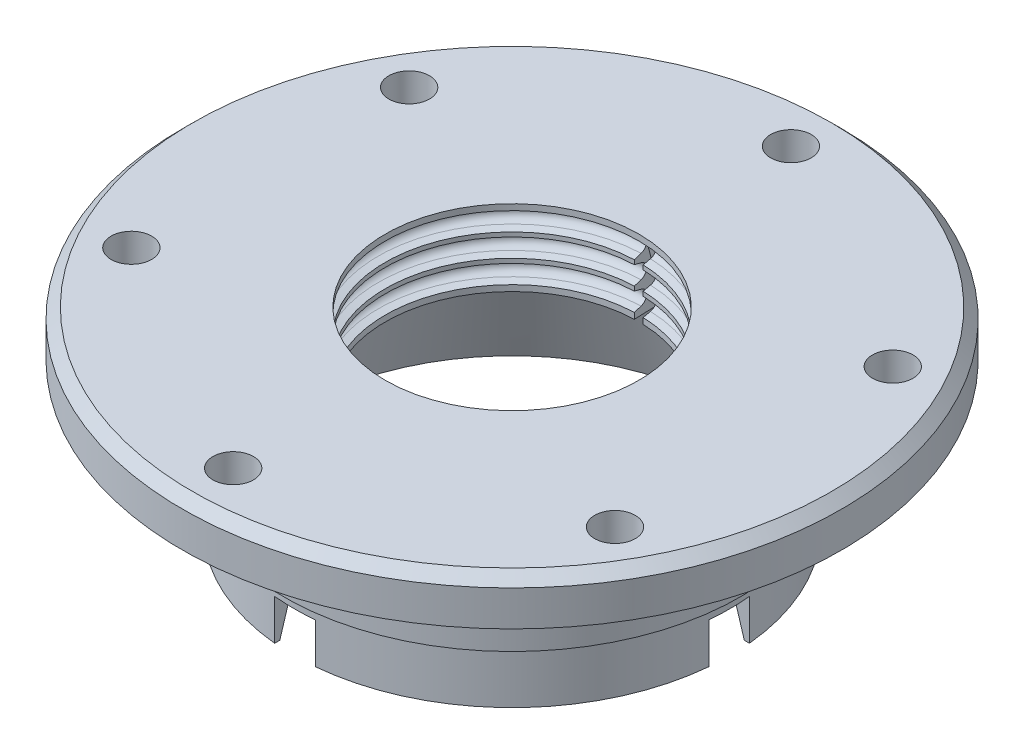
SolidWorks part; units mm, degrees
ref_plane "Front" through (0, 0, 0) normal (0, 0, 1) x (1, 0, 0)
ref_plane "Top" through (0, 0, 0) normal (0, 1, 0) x (1, 0, 0)
ref_plane "Right" through (0, 0, 0) normal (1, 0, 0) x (0, 0, -1)
sketch "Sketch1" plane through (0, 0, 0) normal (0, 0, 1) x (1, 0, 0)
  line L0 (-43, 0) -> (-43, 11)
  line L1 (-43, 11) -> (-45, 11)
  line L2 (-45, 11) -> (-45, 27)
  line L3 (-45, 27) -> (-43, 27)
  line L4 (-43, 27) -> (-43, 29)
  line L5 (-43, 29) -> (-65, 29)
  line L6 (-65, 29) -> (-65, 36)
  line L7 (-63, 38) -> (-25, 38)
  line L8 (-25, 33.1791) -> (-25, 32.3209) construction
  line L9 (-25, 23) -> (-35, 23)
  line L10 (-35, 23) -> (-42, 0)
  line L11 (-42, 0) -> (-43, 0)
  line L12 (-65, 36) -> (-63, 38)
  line L13 (-26, 43.5692) -> (-26, 24.4632) construction
  line L14 (-33.7723, 35) -> (-26, 35) construction
  line L15 (-33.7723, 30.5) -> (-26, 30.5) construction
  line L16 (-33.7723, 26) -> (-26, 26) construction
  line L17 (-26.3882, 36.4489) -> (-25, 36.8209)
  line L18 (-26.3882, 33.5511) -> (-25, 33.1791)
  line L19 (-26.3882, 31.9489) -> (-25, 32.3209)
  line L20 (-26.3882, 24.5511) -> (-25, 24.1791)
  line L21 (-26.5776, 27.3844) -> (-25, 27.8071)
  line L22 (-25, 28.6791) -> (-25, 27.8071) construction
  line L23 (-25, 24.1791) -> (-25, 15.722) construction
  line L24 (-25, 24.1791) -> (-25, 23)
  line L25 (-26.3882, 29.0511) -> (-25, 28.6791)
  line L26 (-25, 40.9901) -> (-25, 36.8209) construction
  line L27 (-25, 33.1791) -> (-25, 32.3209)
  line L28 (-25, 28.6791) -> (-25, 27.8071)
  line L29 (-25, 38) -> (-25, 36.8209)
  line L30 (0, 0) -> (0, 81.7826) construction
  arc A0 (-26.3882, 36.4489) -> (-26.3882, 33.5511) centre (-26, 35) ccw
  arc A1 (-26.3882, 31.9489) -> (-26.3882, 29.0511) centre (-26, 30.5) ccw
  arc A2 (-26.5776, 27.3844) -> (-26.3882, 24.5511) centre (-26, 26) ccw
  point P8 (-65, 38)
  dimension "D19" = 3
  dimension "D20" = 3
  dimension "D21" = 3
  dimension "D2" = 2
  dimension "D3" = 2
  dimension "D4" = 42
  dimension "D5" = 1
  dimension "D6" = 11
  dimension "D7" = 2
  dimension "D8" = 16
  dimension "D9" = 22
  dimension "D10" = 9
  dimension "D11" = 23
  dimension "D12" = 25
  dimension "D16" = 4.5
  dimension "D17" = 7.5
  dimension "D18" = 4.5
  dimension "D22" = 30
  dimension "D23" = 15
  dimension "D24" = 30
  dimension "D25" = 15
  dimension "D26" = 15
  dimension "D27" = 15
  dimension "D28" = 1
revolve "Revolve1" add sketch "Sketch1" angle 360 about L30
fillet "Fillet1" radius 5 1 edges at (0, 23, -35)
sketch "Sketch2" plane through (0, 0, 0) normal (0, 0, 1) x (1, 0, 0)
  line L0 (-43, 0) -> (43, 0) construction
  line L1 (18.079, 0) -> (64.4635, 0)
  line L2 (18.079, 0) -> (18.079, 8)
  line L3 (18.079, 8) -> (64.4635, 8)
  line L4 (64.4635, 0) -> (64.4635, 8)
  line L6 (-21.0009, 0) -> (-54.0544, 0)
  line L7 (-21.0009, 0) -> (-21.0009, 8)
  line L8 (-21.0009, 8) -> (-54.0544, 8)
  line L9 (-54.0544, 0) -> (-54.0544, 8)
  dimension "D1" = 8
  dimension "D2" = 8
extrude "Cut-Extrude1" cut sketch "Sketch2" against normal mid plane 8
sketch "Sketch3" plane through (0, 0, 0) normal (1, 0, 0) x (0, 0, -1)
  line L1 (-63.0026, 8) -> (56.0631, 8)
  line L2 (-63.0026, 8) -> (-63.0026, 0)
  line L3 (-63.0026, 0) -> (56.0631, 0)
  line L4 (56.0631, 8) -> (56.0631, 0)
  dimension "D1" = 8
extrude "Cut-Extrude2" cut sketch "Sketch3" against normal mid plane 8
sketch "Sketch4" plane through (0, 0, 0) normal (1, 0, 0) x (0, 0, -1)
  line L0 (-63, 38) -> (70.5888, 38) construction
  line L1 (70.5888, 35) -> (-27.5, 35) construction
  line L2 (-27.4489, 35.3882) -> (-30.7683, 23)
  line L3 (-26, 54.0152) -> (-26, 36.5) construction
  line L4 (-30.7683, 23) -> (-24.5, 23)
  line L5 (-24.5, 35) -> (-24.5, 23)
  line L6 (-26, 35) -> (-26, 33.5) construction
  line L7 (30.7683, 23) -> (24.5, 23)
  line L8 (0, 0) -> (0, -13.8153) construction
  line L9 (24.5, 35) -> (24.5, 23)
  line L10 (27.4489, 35.3882) -> (30.7683, 23)
  arc A0 (-27.4489, 35.3882) -> (-24.5, 35) centre (-26, 35) ccw
  arc A1 (27.4489, 35.3882) -> (24.5, 35) centre (26, 35) cw
  dimension "D4" = 3
  dimension "D1" = 15
  dimension "D2" = 15
  dimension "D3" = 26
revolve "Cut-Revolve2" cut sketch "Sketch4" angle 4 mid plane about L8
sketch "Sketch5" plane through (0, 0, 0) normal (0, -1, 0) x (1, 0, 0)
  line L0 (0, 0) -> (0, 67.2936) construction
  line L1 (0, 0) -> (91.4154, 0) construction
  line L2 (0, 0) -> (73.9998, 42.7238) construction
  line L3 (0, 0) -> (-75.39, 43.5265) construction
  circle A1 centre (-47.6919, 27.3949) radius 4
  circle A2 centre (0, 55) radius 4
  circle A3 centre (47.6919, 27.3949) radius 4
  circle A4 centre (-47.6919, -27.3949) radius 4
  circle A5 centre (0, -55) radius 4
  circle A6 centre (47.6919, -27.3949) radius 4
  dimension "D4" = 8
  dimension "D5" = 8
  dimension "D6" = 8
  dimension "D1" = 60
  dimension "D2" = 60
extrude "Cut-Extrude3" cut sketch "Sketch5" against normal blind 94
scale "Scale 1" bodies to scale 106 scale about centroid uniform scaling yes scale factor 1.875
